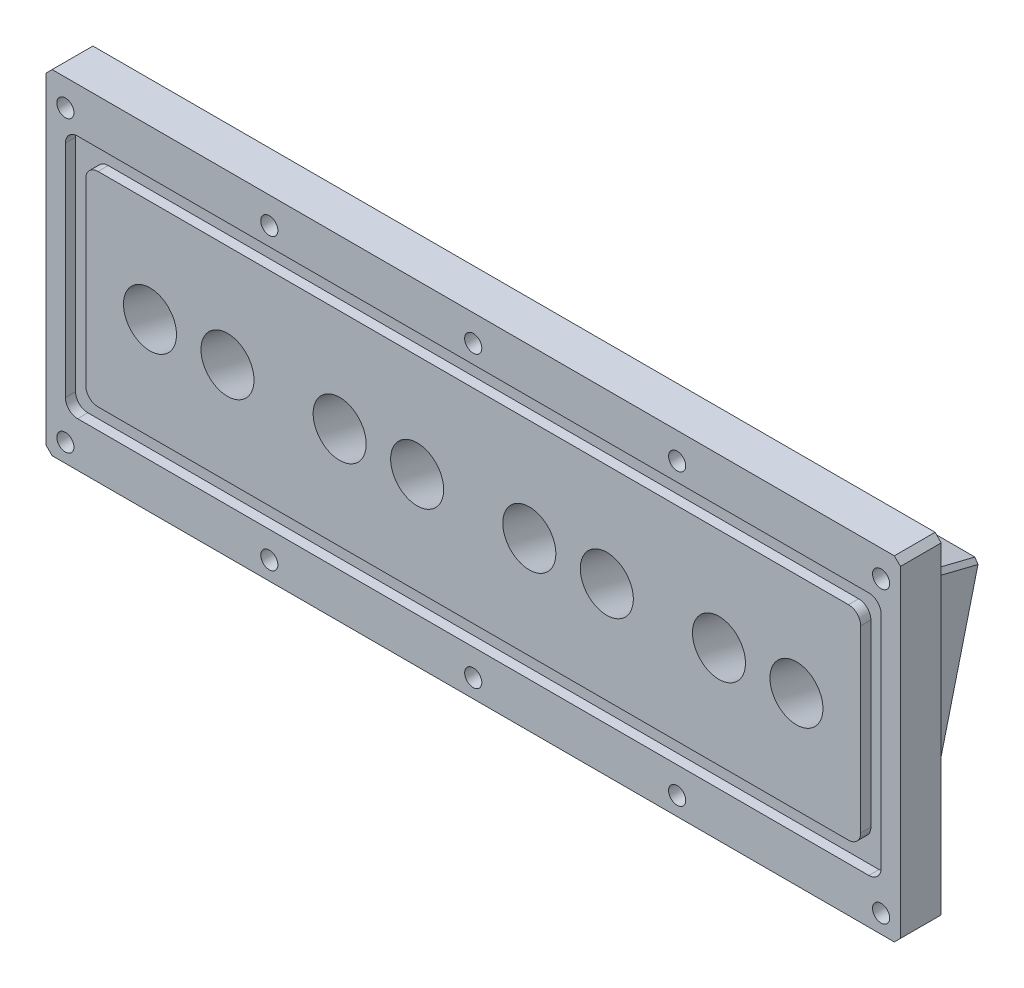
SolidWorks part; units mm, degrees
material "Q235-A"
ref_plane "Front Plane" through (0, 0, 0) normal (0, 0, 1) x (1, 0, 0)
ref_plane "Top Plane" through (0, 0, 0) normal (0, 1, 0) x (1, 0, 0)
ref_plane "Right Plane" through (0, 0, 0) normal (1, 0, 0) x (0, 0, -1)
sketch "Sketch1" plane through (0, 0, 0) normal (0, 0, 1) x (1, 0, 0)
  line L1 (-209.5, -82) -> (209.5, -82)
  line L2 (-209.5, -82) -> (-209.5, 82)
  line L3 (-209.5, 82) -> (209.5, 82)
  line L4 (209.5, -82) -> (209.5, 82)
  line L5 (-209.5, -82) -> (209.5, 82) construction
  line L6 (-209.5, 82) -> (209.5, -82) construction
  point P0 (0, 0)
  dimension "D1" = 419
  dimension "D2" = 164
extrude "Boss-Extrude1" add sketch "Sketch1" along normal blind 20
sketch "Sketch2" plane through (0, 0, 20) normal (0, 0, 1) x (1, 0, 0)
  line L1 (-200, -60) -> (200, -60)
  line L2 (-200, -60) -> (-200, 60)
  line L3 (-200, 60) -> (200, 60)
  line L4 (200, -60) -> (200, 60)
  line L5 (-200, -60) -> (200, 60) construction
  line L6 (-200, 60) -> (200, -60) construction
  line L7 (-190, -50) -> (190, -50)
  line L8 (-190, -50) -> (-190, 50)
  line L9 (-190, 50) -> (190, 50)
  line L10 (190, -50) -> (190, 50)
  line L11 (-190, -50) -> (190, 50) construction
  line L12 (-190, 50) -> (190, -50) construction
  point P0 (0, 0)
  point P6 (0, 0)
  dimension "D1" = 100
  dimension "D2" = 120
  dimension "D3" = 400
  dimension "D4" = 380
extrude "Cut-Extrude1" cut sketch "Sketch2" against normal blind 5
fillet "Fillet1" radius 6 8 edges at (190, 50, 17.5) (200, 60, 17.5) (190, -50, 17.5) (200, -60, 17.5) (-200, -60, 17.5) (-190, -50, 17.5) (-190, 50, 17.5) (-200, 60, 17.5)
chamfer "Chamfer1" distance 3 angle 45 4 edges at (-209.5, -82, 10) (-209.5, 82, 10) (209.5, -82, 10) (209.5, 82, 10)
sketch "Sketch3" plane through (0, 0, 0) normal (0, 0, -1) x (-1, 0, 0)
  line L0 (-206.5, 82) -> (206.5, 82) construction
  line L1 (-209.5, -79) -> (-209.5, 79) construction
  point P0 (-200, 69)
  point P8 (-100, 69)
  point P9 (0, 69)
  point P10 (100, 69)
  point P11 (200, 69)
  point P12 (-100, -73)
  point P13 (0, -73)
  point P14 (100, -73)
  point P15 (200, -73)
  point P16 (-200, -73)
  dimension "D1" = 13
  dimension "D2" = 9.5
  dimension "D3" = 5
  dimension "D4" = 2
hole_wizard "Hole1" positions "Sketch4" profile "Sketch5" legacy end condition through all
sketch "Sketch4" plane through (0, 0, 0) normal (0, 0, -1) x (-1, 0, 0)
  point P0 (-200, 69)
  point P3 (-200, -73)
  point P6 (-100, -73)
  point P9 (0, -73)
  point P12 (100, -73)
  point P15 (200, -73)
  point P18 (200, 69)
  point P21 (100, 69)
  point P24 (0, 69)
  point P27 (-100, 69)
sketch "Sketch5" plane through (200, 69, 0) normal (1, 0, 0) x (0, 1, 0)
  line L0 (0, 0) -> (0, 20)
  line L1 (0, 20) -> (4.2, 20)
  line L2 (4.2, 20) -> (4.2, 11)
  line L3 (4.2, 11) -> (7.5, 11)
  line L4 (7.5, 11) -> (7.5, 0)
  line L5 (7.5, 0) -> (0, 0)
  line L6 (0, 110) -> (0, -10) construction
  dimension "直径" = 8.4
  dimension "深度" = 20
  dimension "柱坑直径" = 15
  dimension "柱坑深度" = 11
ref_plane "Plane1" through (-189.5, 0, 0) normal (-1, 0, 0) x (0, 0, 1)
sketch "Sketch6" plane through (-189.5, 0, 0) normal (-1, 0, 0) x (0, 0, 1)
  line L0 (0, 52.33) -> (-38.51, 42.7325)
  line L1 (0, 79) -> (0, -79) construction
  line L2 (-38.51, 42.7325) -> (-11.8986, -64)
  line L3 (-11.8986, -64) -> (0, -64)
  line L4 (0, -64) -> (0, 52.33)
  line L5 (20, -82) -> (0, -82) construction
  line L6 (20, 79) -> (20, -79) construction
  dimension "D1" = 116.33
  dimension "D2" = 18
  dimension "D3" = 58.51
  dimension "D4" = 110
  dimension "D5" = 14
  dimension "D6" = 11.8986
extrude "Boss-Extrude2" add sketch "Sketch6" against normal blind 379
chamfer "Chamfer2" distance 2 angle 45 4 edges at (189.5, -64, -5.9493) (189.5, 47.5313, -19.255) (-189.5, -64, -5.9493) (-189.5, 47.5313, -19.255)
sketch "Sketch7" plane through (0, -6.5387, -26.2253) normal (0, -0.2419, -0.9703) x (-1, 0, 0)
  line L0 (-187.5, 50.7756) -> (187.5, 50.7756) construction
  line L1 (209.5, 76.6534) -> (209.5, -76.6534) construction
  line L2 (16.5, -49.9244) -> (16.5, 40.0756)
  line L3 (109.5, -49.9244) -> (169.5, -49.9244)
  line L4 (109.5, -49.9244) -> (109.5, 40.0756)
  line L5 (109.5, 40.0756) -> (169.5, 40.0756)
  line L6 (169.5, -49.9244) -> (169.5, 40.0756)
  line L7 (109.5, -49.9244) -> (169.5, 40.0756) construction
  line L8 (109.5, 40.0756) -> (169.5, -49.9244) construction
  line L9 (16.5, -49.9244) -> (76.5, -49.9244)
  line L10 (76.5, -49.9244) -> (76.5, 40.0756)
  line L11 (16.5, 40.0756) -> (76.5, 40.0756)
  line L12 (-76.5, -49.9244) -> (-76.5, 40.0756)
  line L13 (-76.5, -49.9244) -> (-16.5, -49.9244)
  line L14 (-16.5, -49.9244) -> (-16.5, 40.0756)
  line L15 (-76.5, 40.0756) -> (-16.5, 40.0756)
  line L16 (-169.5, -49.9244) -> (-169.5, 40.0756)
  line L17 (-169.5, -49.9244) -> (-109.5, -49.9244)
  line L18 (-109.5, -49.9244) -> (-109.5, 40.0756)
  line L19 (-169.5, 40.0756) -> (-109.5, 40.0756)
  point P0 (158.5, -4.9244)
  point P3 (120.5011, -5.2142)
  point P6 (139.5, -4.9244)
  point P8 (65.5, -4.9244)
  point P9 (27.5011, -5.2142)
  point P10 (-27.5, -4.9244)
  point P11 (-65.4989, -5.2142)
  point P12 (-120.5, -4.9244)
  point P13 (-158.4989, -5.2142)
  dimension "D1" = 55.7
  dimension "D2" = 51
  dimension "D3" = 38
  dimension "D5" = 40
  dimension "D6" = 60
  dimension "D7" = 90
  dimension "D8" = 10.7
  dimension "D4" = 4
  dimension "D9" = 4
hole_wizard "Hole2" positions "Sketch8" profile "Sketch9" legacy end condition through all
sketch "Sketch8" plane through (0, -6.5387, -26.2253) normal (0, -0.2419, -0.9703) x (-1, 0, 0)
  point P0 (158.5, -4.9244)
  point P3 (120.5011, -5.2142)
  point P6 (65.5, -4.9244)
  point P9 (27.5011, -5.2142)
  point P12 (-27.5, -4.9244)
  point P15 (-65.4989, -5.2142)
  point P18 (-120.5, -4.9244)
  point P21 (-158.4989, -5.2142)
sketch "Sketch9" plane through (-158.5, -11.3169, -25.034) normal (1, 0, 0) x (0, 0.9703, -0.2419)
  line L0 (0, 0) -> (0, 66.2717)
  line L1 (0, 66.2717) -> (13, 66.2717)
  line L2 (13, 66.2717) -> (13, 0)
  line L3 (13, 0) -> (0, 0)
  line L4 (0, 110) -> (0, -10) construction
  dimension "直径" = 26
  dimension "深度" = 66.2717
hole_wizard "M6 Tapped Hole1" positions "Sketch10" profile "Sketch11" tap size "M6" standard "GB"
sketch "Sketch10" plane through (0, -6.5387, -26.2253) normal (0, -0.2419, -0.9703) x (-1, 0, 0)
  point P0 (-169.5, 40.0756)
  point P3 (-109.5, 40.0756)
  point P6 (-76.5, 40.0756)
  point P9 (-16.5, 40.0756)
  point P12 (16.5, 40.0756)
  point P15 (76.5, 40.0756)
  point P18 (109.5, 40.0756)
  point P21 (169.5, 40.0756)
  point P24 (169.5, -49.9244)
  point P27 (109.5, -49.9244)
  point P30 (76.5, -49.9244)
  point P33 (16.5, -49.9244)
  point P36 (-16.5, -49.9244)
  point P39 (-76.5, -49.9244)
  point P42 (-109.5, -49.9244)
  point P45 (-169.5, -49.9244)
sketch "Sketch11" plane through (169.5, 32.3465, -35.9205) normal (1, 0, 0) x (0, 0.9703, -0.2419)
  line L0 (0, 0) -> (0, 13.5022)
  line L1 (0, 13.5022) -> (2.5, 12)
  line L2 (2.5, 12) -> (2.5, 0)
  line L5 (2.5, 0) -> (0, 0)
  line L10 (0, 13.5022) -> (-2.5, 12) construction
  line L11 (0, -6.35) -> (0, 107.95) construction
  dimension "螺纹孔钻头直径" = 5
  dimension "螺纹孔钻头深度" = 12
  dimension "导头角度" = 118
cosmetic thread "Cosmetic Thread1" parameters "D1"=12, "D2"=6
cosmetic thread "Cosmetic Thread2" parameters "D1"=12, "D2"=6
cosmetic thread "Cosmetic Thread3" parameters "D1"=12, "D2"=6
cosmetic thread "Cosmetic Thread4" parameters "D1"=12, "D2"=6
cosmetic thread "Cosmetic Thread5" parameters "D1"=12, "D2"=6
cosmetic thread "Cosmetic Thread6" parameters "D1"=12, "D2"=6
cosmetic thread "Cosmetic Thread7" parameters "D1"=12, "D2"=6
cosmetic thread "Cosmetic Thread8" parameters "D1"=12, "D2"=6
cosmetic thread "Cosmetic Thread9" parameters "D1"=12, "D2"=6
cosmetic thread "Cosmetic Thread10" parameters "D1"=12, "D2"=6
cosmetic thread "Cosmetic Thread11" parameters "D1"=12, "D2"=6
cosmetic thread "Cosmetic Thread12" parameters "D1"=12, "D2"=6
cosmetic thread "Cosmetic Thread13" parameters "D1"=12, "D2"=6
cosmetic thread "Cosmetic Thread14" parameters "D1"=12, "D2"=6
cosmetic thread "Cosmetic Thread15" parameters "D1"=12, "D2"=6
cosmetic thread "Cosmetic Thread16" parameters "D1"=12, "D2"=6
sketch "Sketch12" plane through (0, -6.5387, -26.2253) normal (0, -0.2419, -0.9703) x (-1, 0, 0)
  line L0 (209.5, 76.6534) -> (209.5, -76.6534) construction
  line L1 (-179.5, 34.0796) -> (179.5, 34.0796)
  line L2 (-179.5, 34.0796) -> (-179.5, -43.9204)
  line L3 (-179.5, -43.9204) -> (179.5, -43.9204)
  line L4 (179.5, 34.0796) -> (179.5, -43.9204)
  line L5 (-187.5, 50.7796) -> (187.5, 50.7796) construction
  dimension "D1" = 359
  dimension "D2" = 30
  dimension "D3" = 78
  dimension "D4" = 16.7
extrude "Cut-Extrude2" cut sketch "Sketch12" against normal blind 15
fillet "Fillet2" radius 6 4 edges at (-179.5, -47.3401, -8.3228) (-179.5, 28.343, -27.1927) (179.5, -47.3401, -8.3228) (179.5, 28.343, -27.1927)
